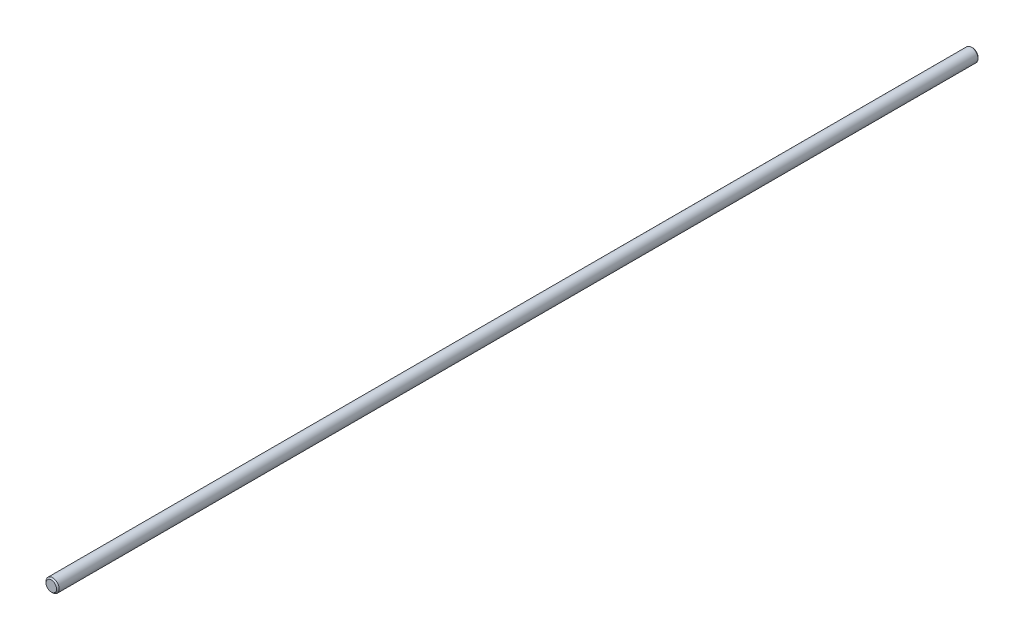
from build123d import *

# Parameters (mm, degrees)
SKETCH1_R           = 5
BOSS_EXTRUDE1_DEPTH = 350
CHAMFER1_SIZE       = 1


with BuildPart() as part:
    # Sketch1 → Boss-Extrude1 (new, symmetric)
    with BuildSketch(Plane.XY):
        Circle(SKETCH1_R)
    extrude(amount=BOSS_EXTRUDE1_DEPTH, both=True)

    # Chamfer1
    chamfer1_edges = [part.edges().sort_by_distance(p)[0] for p in [
        (-5, 0, -350),
        (-5, 0, 350),
    ]]
    chamfer(chamfer1_edges, length=CHAMFER1_SIZE)


solid = part.part
